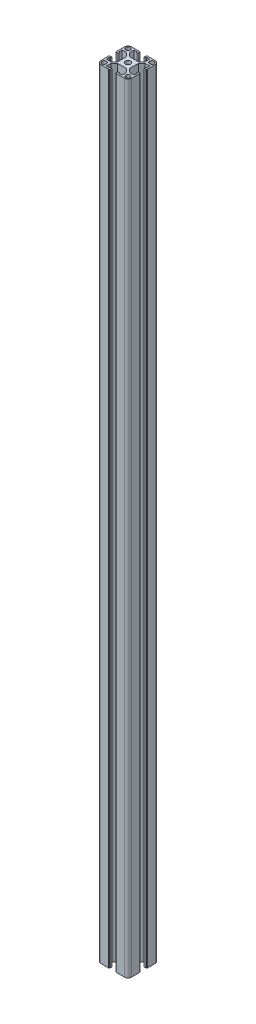
SolidWorks part; units mm, degrees
ref_plane "主视基准图" through (0, 0, 0) normal (0, 0, 1) x (1, 0, 0)
ref_plane "上视基准图" through (0, 0, 0) normal (0, 1, 0) x (1, 0, 0)
ref_plane "右视基准图" through (0, 0, 0) normal (1, 0, 0) x (0, 0, -1)
sketch "草图1" plane through (0, 0, 0) normal (0, 0, 1) x (1, 0, 0)
  line L0 (0, 0) -> (0, 1013)
  dimension "D1" = 1013
other "结构构件1"
ref_plane "基准面1" through (0, 0, 0) normal (0, 1, 0) x (-1, 0, 0)
sketch "Sketch16" plane through (0, 0, 0) normal (0, 1, 0) x (-1, 0, 0)
  line L0 (-5.1, 20) -> (-5.1, 19.5)
  line L1 (-5.1, 19.5) -> (-4.1, 19.5)
  line L2 (-4.1, 19.5) -> (-4.1, 17)
  line L3 (-6.1, 18) -> (-10.3, 18)
  line L4 (-15.5, -20) -> (-5.1, -20)
  line L5 (-20, -15.5) -> (-20, -5.1)
  line L6 (15.5, 20) -> (5.1, 20)
  line L7 (20, 15.5) -> (20, 5.1)
  line L8 (0, 14.8756) -> (0, 0) construction
  line L9 (0, 0) -> (14.1675, 0) construction
  line L10 (-10.3, 18) -> (-10.3, 12)
  line L11 (-10.3, 12) -> (-6, 7.7)
  line L12 (-6, 7.7) -> (6, 7.7)
  line L13 (10.3, 12) -> (6, 7.7)
  line L14 (10.3, 18) -> (10.3, 12)
  line L15 (6.1, 18) -> (10.3, 18)
  line L16 (4.1, 19.5) -> (4.1, 17)
  line L17 (5.1, 19.5) -> (4.1, 19.5)
  line L18 (5.1, 20) -> (5.1, 19.5)
  line L19 (-5.1, 20) -> (-15.5, 20)
  line L20 (20, 5.1) -> (19.5, 5.1)
  line L21 (0, 0) -> (-15.5563, 15.5563) construction
  line L22 (0, 0) -> (-15.5563, -15.5563) construction
  line L25 (19.5, 5.1) -> (19.5, 4.1)
  line L26 (19.5, 4.1) -> (17, 4.1)
  line L27 (17, 6.1) -> (17, 4.1)
  line L28 (18, 6.1) -> (17, 6.1)
  line L29 (18, 6.1) -> (18, 10.3)
  line L30 (18, 10.3) -> (12, 10.3)
  line L31 (12, 10.3) -> (7.7, 6)
  line L32 (7.7, 6) -> (7.7, -6)
  line L33 (12, -10.3) -> (7.7, -6)
  line L34 (18, -10.3) -> (12, -10.3)
  line L35 (18, -6.1) -> (18, -10.3)
  line L36 (18, -6.1) -> (17, -6.1)
  line L37 (17, -4.1) -> (17, -6.1)
  line L38 (19.5, -4.1) -> (17, -4.1)
  line L39 (19.5, -5.1) -> (19.5, -4.1)
  line L40 (20, -5.1) -> (19.5, -5.1)
  line L41 (5.1, -20) -> (5.1, -19.5)
  line L42 (5.1, -19.5) -> (4.1, -19.5)
  line L43 (4.1, -19.5) -> (4.1, -17)
  line L44 (6.1, -17) -> (4.1, -17)
  line L45 (6.1, -18) -> (6.1, -17)
  line L46 (6.1, -18) -> (10.3, -18)
  line L47 (10.3, -18) -> (10.3, -12)
  line L48 (10.3, -12) -> (6, -7.7)
  line L49 (6, -7.7) -> (-6, -7.7)
  line L50 (-10.3, -12) -> (-6, -7.7)
  line L51 (-10.3, -18) -> (-10.3, -12)
  line L52 (-6.1, -18) -> (-10.3, -18)
  line L53 (-6.1, -18) -> (-6.1, -17)
  line L54 (-4.1, -17) -> (-6.1, -17)
  line L55 (-4.1, -19.5) -> (-4.1, -17)
  line L56 (-5.1, -19.5) -> (-4.1, -19.5)
  line L57 (-5.1, -20) -> (-5.1, -19.5)
  line L58 (-20, -5.1) -> (-19.5, -5.1)
  line L59 (5.1, -20) -> (15.5, -20)
  line L60 (-20, 5.1) -> (-20, 15.5)
  line L61 (-19.5, -5.1) -> (-19.5, -4.1)
  line L62 (-6.1, 18) -> (-6.1, 17)
  line L63 (-6.1, 17) -> (-4.1, 17)
  line L64 (6.1, 18) -> (6.1, 17)
  line L65 (4.1, 17) -> (6.1, 17)
  line L66 (-19.5, -4.1) -> (-17, -4.1)
  line L71 (-17, -6.1) -> (-17, -4.1)
  line L72 (-18, -6.1) -> (-17, -6.1)
  line L73 (-18, -6.1) -> (-18, -10.3)
  line L74 (-18, -10.3) -> (-12, -10.3)
  line L75 (-12, -10.3) -> (-7.7, -6)
  line L76 (-7.7, -6) -> (-7.7, 6)
  line L77 (-12, 10.3) -> (-7.7, 6)
  line L78 (-18, 10.3) -> (-12, 10.3)
  line L79 (-18, 6.1) -> (-18, 10.3)
  line L80 (-18, 6.1) -> (-17, 6.1)
  line L81 (-17, 4.1) -> (-17, 6.1)
  line L82 (-19.5, 4.1) -> (-17, 4.1)
  line L83 (-19.5, 5.1) -> (-19.5, 4.1)
  line L84 (-20, 5.1) -> (-19.5, 5.1)
  line L85 (20, -5.1) -> (20, -15.5)
  circle A0 centre (0, 0) radius 3.4
  arc A1 (-20, 15.5) -> (-15.5, 20) centre (-15.5, 15.5) cw
  arc A2 (20, 15.5) -> (15.5, 20) centre (15.5, 15.5) ccw
  arc A3 (-15.5, -20) -> (-20, -15.5) centre (-15.5, -15.5) cw
  arc A4 (15.5, -20) -> (20, -15.5) centre (15.5, -15.5) ccw
  circle A5 centre (-15.5563, 15.5563) radius 3
  circle A6 centre (15.5563, 15.5563) radius 3
  circle A7 centre (15.5563, -15.5563) radius 3
  circle A8 centre (-15.5563, -15.5563) radius 3
  point P2 (0, 10)
  point P3 (0, 0)
  point P4 (0, 0)
  point P5 (-20, -20)
  point P6 (20, -20)
  point P7 (20, 20)
  point P8 (-20, 20)
  point P36 (-20, 20)
  point P39 (20, 20)
  dimension "D1" = 20.6
  dimension "D2" = 40
  dimension "D3" = 8.2
  dimension "D4" = 10.2
  dimension "D5" = 12.3
  dimension "D6" = 6.8
  dimension "D7" = 4.5
  dimension "D8" = 45
  dimension "D12" = 6
  dimension "D13" = 22
  dimension "D9" = 0.5
  dimension "D10" = 2
  dimension "D11" = 12
  dimension "D16" = 3
  dimension "D17" = 2
